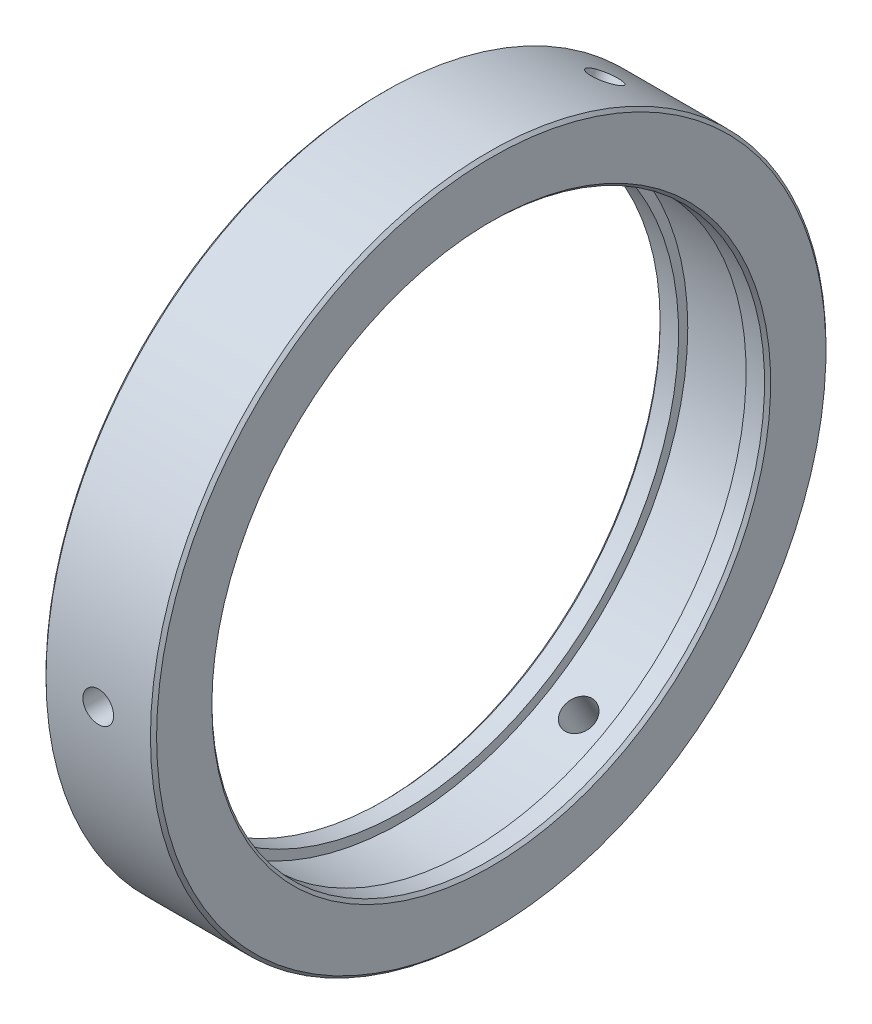
SolidWorks part; units mm, degrees
material "HT200"
ref_plane "Front Plane" through (0, 0, 0) normal (0, 0, 1) x (1, 0, 0)
ref_plane "Top Plane" through (0, 0, 0) normal (0, 1, 0) x (1, 0, 0)
ref_plane "Right Plane" through (0, 0, 0) normal (1, 0, 0) x (0, 0, -1)
sketch "Sketch2" plane through (0, 0, 0) normal (0, 0, 1) x (1, 0, 0)
  line L0 (-18, 90) -> (-18, 110)
  line L1 (-18, 110) -> (18, 110)
  line L2 (18, 110) -> (18, 90)
  line L3 (18, 90) -> (11, 90)
  line L4 (11, 90) -> (11, 93)
  line L5 (11, 93) -> (-11, 93)
  line L6 (-11, 93) -> (-11, 90)
  line L7 (-11, 90) -> (-18, 90)
  line L8 (-24.3325, 0) -> (74.5974, 0) construction
  dimension "D1" = 36
  dimension "D2" = 7
  dimension "D3" = 22
  dimension "D4" = 18
  dimension "D5" = 110
  dimension "D6" = 93
  dimension "D7" = 90
revolve "Revolve1" add sketch "Sketch2" angle 360 about L8
chamfer "Chamfer1" distance 1 angle 45 4 edges at (-18, 0, 110) (-18, 0, 90) (18, 0, 90) (18, 0, 110)
hole_wizard "Hole1" positions "3DSketch1" profile "Sketch4" legacy
sketch3d "3DSketch1"
  point P0 (0, 0, 110)
  dimension "D1" = 18
sketch "Sketch4" plane through (0, 0, 110) normal (1, 0, 0) x (0, -1, 0)
  line L0 (0, 0) -> (0, 18)
  line L1 (0, 18) -> (5, 18)
  line L2 (5, 18) -> (5, 0)
  line L3 (5, 0) -> (0, 0)
  line L4 (0, 110) -> (0, -10) construction
  dimension "直径" = 10
  dimension "深度" = 18
pattern_circular "CirPattern1" count 3 over 360 about axis through (17, 0, 0) along (-1, 0, 0) of "Hole1"
